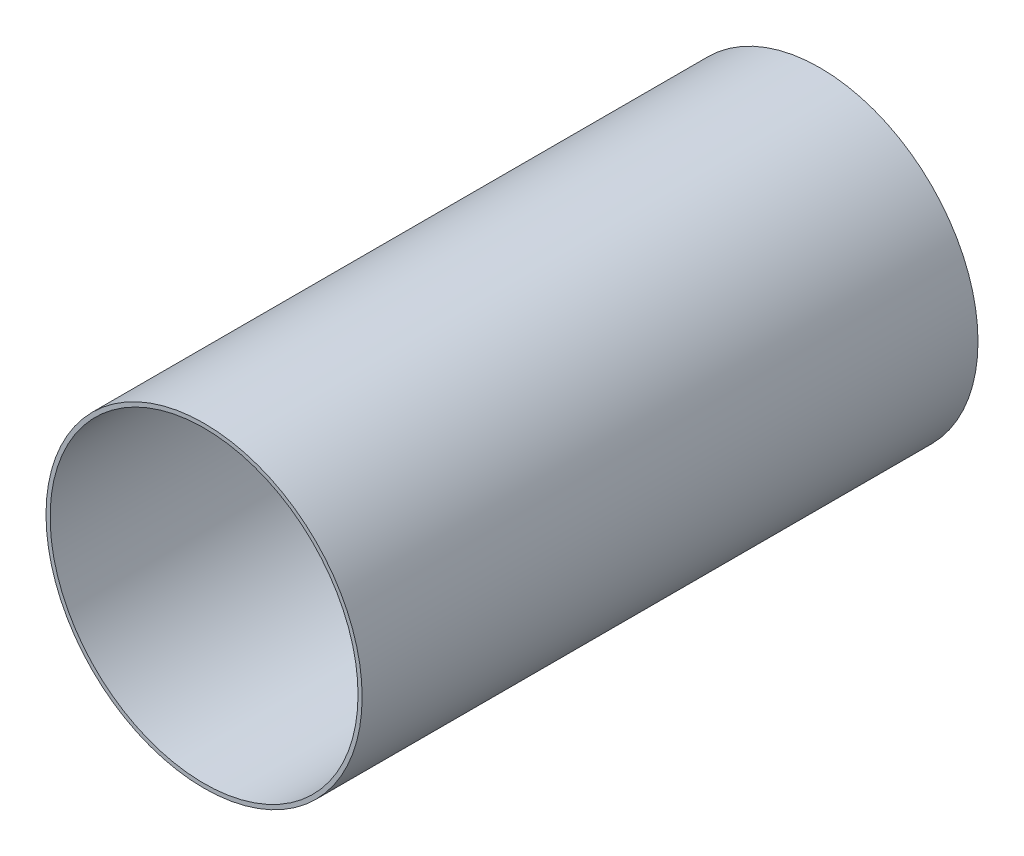
from build123d import *

# Parameters (mm, degrees)
SKETCH1_R           = 77
SKETCH1_R_2         = 75
BOSS_EXTRUDE1_DEPTH = 300


with BuildPart() as part:
    # Sketch1 → Boss-Extrude1 (new body)
    with BuildSketch(Plane.XY):
        Circle(SKETCH1_R)
        Circle(SKETCH1_R_2, mode=Mode.SUBTRACT)
    extrude(amount=BOSS_EXTRUDE1_DEPTH)


solid = part.part
